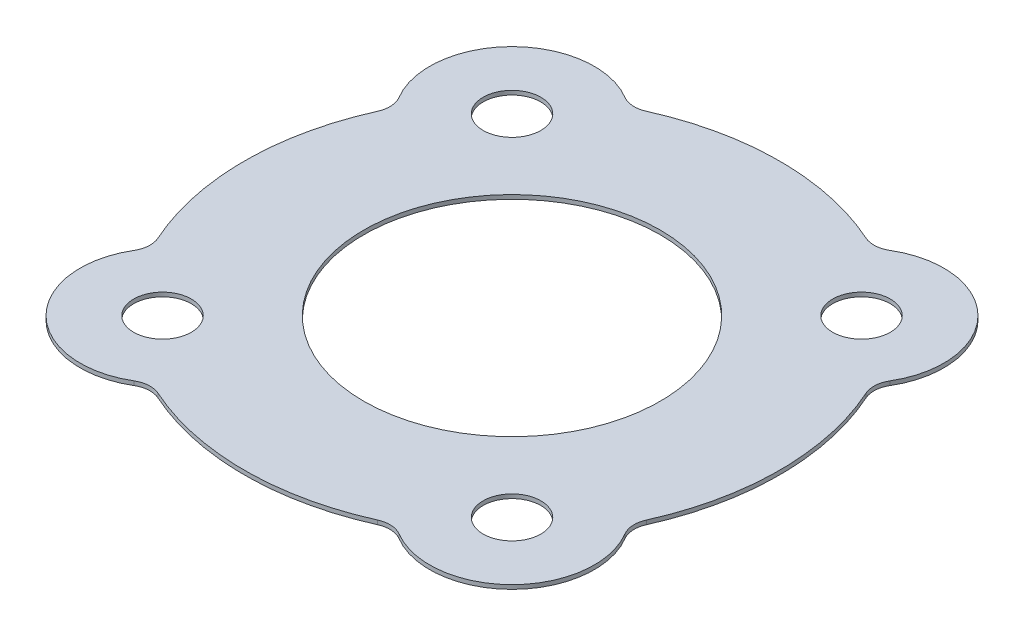
from build123d import *

# Parameters (mm, degrees)
SKETCH1_R           = 10
SKETCH1_R_2         = 32.5
BOSS_EXTRUDE1_DEPTH = 0.5
SKETCH2_R           = 18
SKETCH2_R_2         = 3.5
CUT_EXTRUDE1_DEPTH  = 50
FILLET1_R           = 3


with BuildPart() as part:
    # Sketch1 → Boss-Extrude1 (new body)
    with BuildSketch(Plane(origin=(0, 0, 0), x_dir=(1, 0, 0), z_dir=(0, 1, 0))):
        with Locations((-21.213203436, -21.213203436)):
            Circle(SKETCH1_R)
        Circle(SKETCH1_R_2)
        with Locations((21.213203436, -21.213203436)):
            Circle(SKETCH1_R)
        with Locations((21.213203436, 21.213203436)):
            Circle(SKETCH1_R)
        with Locations((-21.213203436, 21.213203436)):
            Circle(SKETCH1_R)
    extrude(amount=BOSS_EXTRUDE1_DEPTH)

    # Sketch2 → Cut-Extrude1 (cut)
    with BuildSketch(Plane(origin=(0, 0.5, 0), x_dir=(1, 0, 0), z_dir=(0, 1, 0))):
        with Locations(Location((0, 0, 0), (0, 0, 270))):
            Circle(SKETCH2_R)
        with Locations(Location((21.213203436, 21.213203436, 0), (0, 0, 270))):
            Circle(SKETCH2_R_2)
        with Locations(Location((21.213203436, -21.213203436, 0), (0, 0, 270))):
            Circle(SKETCH2_R_2)
        with Locations(Location((-21.213203436, -21.213203436, 0), (0, 0, 270))):
            Circle(SKETCH2_R_2)
        with Locations(Location((-21.213203436, 21.213203436, 0), (0, 0, 270))):
            Circle(SKETCH2_R_2)
    extrude(amount=-CUT_EXTRUDE1_DEPTH, mode=Mode.SUBTRACT)

    # Fillet1
    fillet1_edges = [part.edges().sort_by_distance(p)[0] for p in [
        (-28.916041247, 0.25, -14.836190839),
        (-14.836190839, 0.25, -28.916041247),
        (14.836190839, 0.25, -28.916041247),
        (28.916041247, 0.25, -14.836190839),
        (28.916041247, 0.25, 14.836190839),
        (14.836190839, 0.25, 28.916041247),
        (-14.836190839, 0.25, 28.916041247),
        (-28.916041247, 0.25, 14.836190839),
    ]]
    fillet(fillet1_edges, radius=FILLET1_R)


solid = part.part
